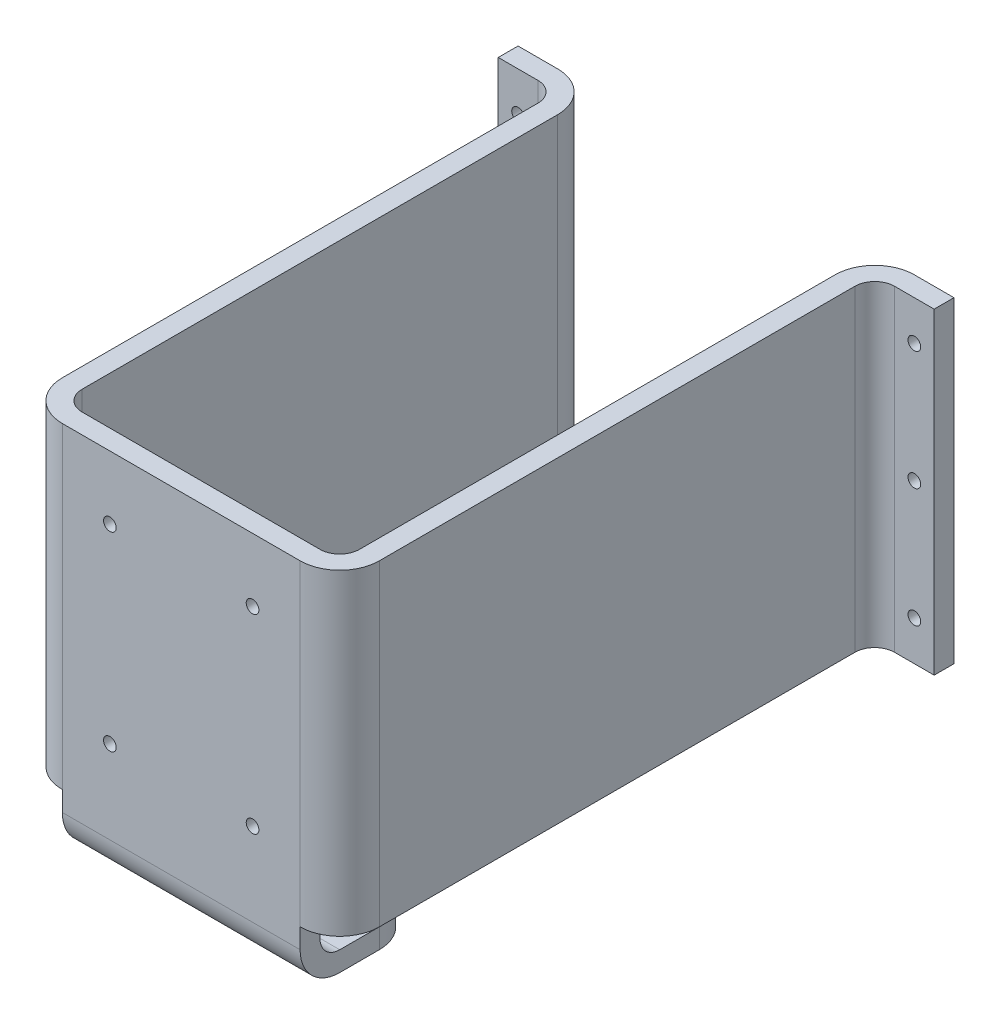
from build123d import *

# Parameters (mm, degrees)
BOSS_EXTRUDE1_DEPTH = 80
SKETCH2_W           = 5
SKETCH2_H           = 80
BOSS_EXTRUDE2_DEPTH = 15
SKETCH3_W           = 5
SKETCH3_H           = 80
BOSS_EXTRUDE3_DEPTH = 15
FILLET1_R           = 10
FILLET2_R           = 5
SKETCH4_W           = 60
SKETCH4_H           = 5
BOSS_EXTRUDE4_DEPTH = 15
SKETCH5_W           = 60
SKETCH5_H           = 5
BOSS_EXTRUDE5_DEPTH = 25
FILLET3_R           = 5
FILLET4_R           = 10
SKETCH6_R           = 1.6
CUT_EXTRUDE1_DEPTH  = 10
FILLET5_R           = 10
SKETCH7_R           = 1.6
CUT_EXTRUDE2_DEPTH  = 188.149672722
SKETCH8_R           = 1.6
CUT_EXTRUDE3_DEPTH  = 184.439363278


with BuildPart() as part:
    # Sketch1 → Boss-Extrude1 (new body)
    with BuildSketch(Plane(origin=(0, 0, 0), x_dir=(1, 0, 0), z_dir=(0, 1, 0))):
        Polygon((0, 0), (0, 134.306122449), (5, 134.306122449), (5, -0.693877551), (75, -0.693877551), (75, 134.306122449), (80, 134.306122449), (80, -5.693877551), (35.857142857, -5.693877551), (0, -5.693877551), align=None)
    extrude(amount=BOSS_EXTRUDE1_DEPTH)

    # Sketch2 → Boss-Extrude2 (add)
    with BuildSketch(Plane(origin=(80, 0, 0), x_dir=(0, 0, -1), z_dir=(1, 0, 0))):
        with Locations((131.806122449, 40)):
            Rectangle(SKETCH2_W, SKETCH2_H)
    extrude(amount=BOSS_EXTRUDE2_DEPTH)

    # Sketch3 → Boss-Extrude3 (add)
    with BuildSketch(Plane.ZY):
        with Locations((-131.806122449, 40)):
            Rectangle(SKETCH3_W, SKETCH3_H)
    extrude(amount=BOSS_EXTRUDE3_DEPTH)

    # Fillet1
    fillet1_edges = [part.edges().sort_by_distance(p)[0] for p in [
        (5, 40, -134.306122449),
        (75, 40, -134.306122449),
        (80, 40, 5.693877551),
        (0, 40, 5.693877551),
    ]]
    fillet(fillet1_edges, radius=FILLET1_R)

    # Fillet2
    fillet2_edges = [part.edges().sort_by_distance(p)[0] for p in [
        (5, 40, 0.693877551),
        (75, 40, 0.693877551),
        (80, 40, -129.306122449),
        (0, 40, -129.306122449),
    ]]
    fillet(fillet2_edges, radius=FILLET2_R)

    # Sketch4 → Boss-Extrude4 (add)
    with BuildSketch(Plane.XZ):
        with Locations((40, 3.193877551)):
            Rectangle(SKETCH4_W, SKETCH4_H)
    extrude(amount=BOSS_EXTRUDE4_DEPTH)

    # Sketch5 → Boss-Extrude5 (add)
    with BuildSketch(Plane(origin=(0, 0, 0.693877551), x_dir=(-1, 0, 0), z_dir=(0, 0, -1))):
        with Locations((-40, -12.5)):
            Rectangle(SKETCH5_W, SKETCH5_H)
    extrude(amount=BOSS_EXTRUDE5_DEPTH)

    # Fillet3
    fillet3_edges = [part.edges().sort_by_distance(p)[0] for p in [
        (40, -10, 0.693877551),
    ]]
    fillet(fillet3_edges, radius=FILLET3_R)

    # Fillet4
    fillet4_edges = [part.edges().sort_by_distance(p)[0] for p in [
        (40, -15, 5.693877551),
    ]]
    fillet(fillet4_edges, radius=FILLET4_R)

    # Sketch6 → Cut-Extrude1 (cut)
    with BuildSketch(Plane.XZ.offset(15)):
        with Locations(Location((17.5, -16.306122449, 0), (0, 0, 270))):
            Circle(SKETCH6_R)
        with Locations(Location((62.5, -16.306122449, 0), (0, 0, 270))):
            Circle(SKETCH6_R)
    extrude(amount=-CUT_EXTRUDE1_DEPTH, mode=Mode.SUBTRACT)

    # Fillet5
    fillet5_edges = [part.edges().sort_by_distance(p)[0] for p in [
        (70, -12.5, -24.306122449),
        (10, -12.5, -24.306122449),
    ]]
    fillet(fillet5_edges, radius=FILLET5_R)

    # Sketch7 → Cut-Extrude2 (cut, through all)
    with BuildSketch(Plane.XY.offset(5.693877551)):
        with Locations((22, 64)):
            Circle(SKETCH7_R)
        with Locations((58, 64)):
            Circle(SKETCH7_R)
        with Locations((58, 16)):
            Circle(SKETCH7_R)
        with Locations((22, 16)):
            Circle(SKETCH7_R)
    extrude(amount=-CUT_EXTRUDE2_DEPTH, mode=Mode.SUBTRACT)

    # Sketch8 → Cut-Extrude3 (cut, through all)
    with BuildSketch(Plane.XY.offset(-129.306122449)):
        with Locations((-10, 70)):
            Circle(SKETCH8_R)
        with Locations((-10, 40)):
            Circle(SKETCH8_R)
        with Locations((-10, 10)):
            Circle(SKETCH8_R)
        with Locations((90, 70)):
            Circle(SKETCH8_R)
        with Locations((90, 40)):
            Circle(SKETCH8_R)
        with Locations((90, 10)):
            Circle(SKETCH8_R)
    extrude(amount=-CUT_EXTRUDE3_DEPTH, mode=Mode.SUBTRACT)


solid = part.part
